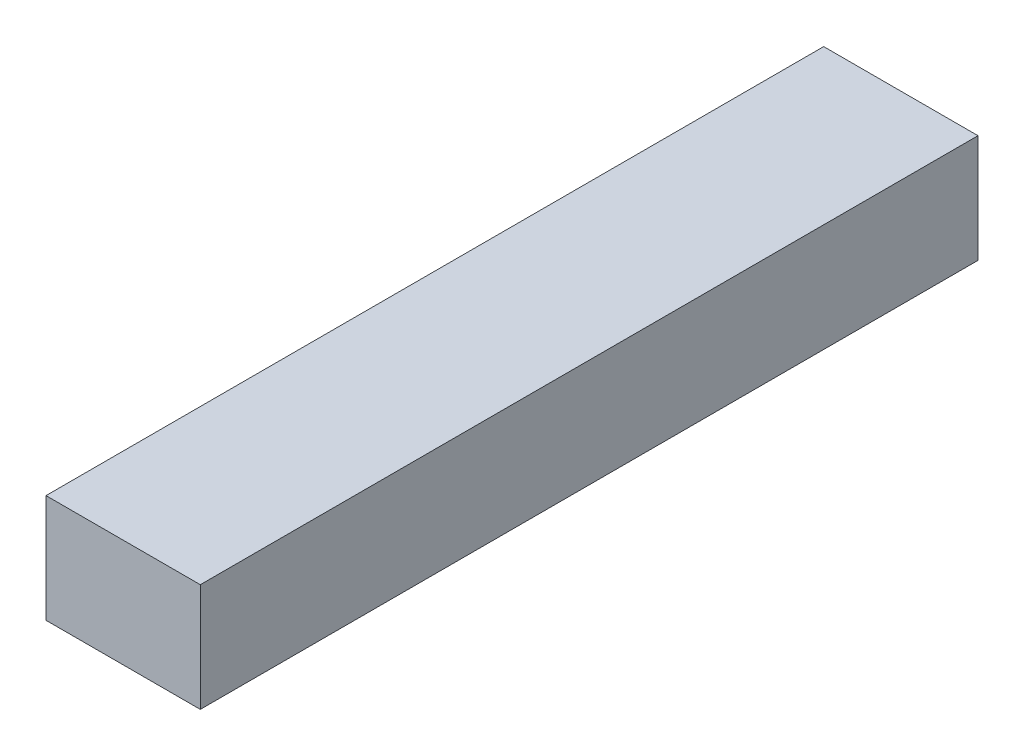
SolidWorks part; units mm, degrees
material "Q345B"
ref_plane "Front Plane" through (0, 0, 0) normal (0, 0, 1) x (1, 0, 0)
ref_plane "Top Plane" through (0, 0, 0) normal (0, 1, 0) x (1, 0, 0)
ref_plane "Right Plane" through (0, 0, 0) normal (1, 0, 0) x (0, 0, -1)
sketch "Sketch2" plane through (0, 0, 0) normal (0, 1, 0) x (1, 0, 0)
  line L0 (-131.395, 0) -> (113.7022, 0) construction
  line L1 (0, 164.1787) -> (0, -121.5078) construction
  line L3 (-12.5, 63) -> (12.5, 63)
  line L4 (-12.5, 63) -> (-12.5, -63)
  line L5 (-12.5, -63) -> (12.5, -63)
  line L6 (12.5, 63) -> (12.5, -63)
  dimension "D1" = 126
  dimension "D2" = 25
  dimension "D3" = 12.5
extrude "Boss-Extrude1" add sketch "Sketch2" along normal mid plane 17.5
